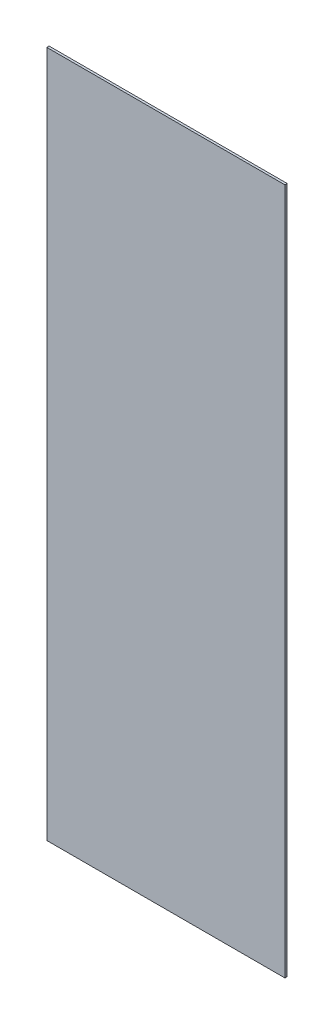
SolidWorks part; units mm, degrees
material "PMMA(有机玻璃)"
ref_plane "前视" through (0, 0, 0) normal (0, 0, 1) x (1, 0, 0)
ref_plane "上视" through (0, 0, 0) normal (0, 1, 0) x (1, 0, 0)
ref_plane "右视" through (0, 0, 0) normal (1, 0, 0) x (0, 0, -1)
sketch "草图1" plane through (0, 0, 0) normal (0, 0, 1) x (1, 0, 0)
  line L1 (-258.5, 745.5) -> (258.5, 745.5)
  line L2 (-258.5, 745.5) -> (-258.5, -745.5)
  line L3 (-258.5, -745.5) -> (258.5, -745.5)
  line L4 (258.5, 745.5) -> (258.5, -745.5)
  line L5 (-258.5, 745.5) -> (258.5, -745.5) construction
  line L6 (-258.5, -745.5) -> (258.5, 745.5) construction
  point P0 (0, 0)
  dimension "D1" = 1491
  dimension "D2" = 517
extrude "凸台-拉伸1" add sketch "草图1" along normal blind 5
hole_wizard "M5 间隙孔1" positions "草图3" profile "草图2" hole size "M5" standard "GB"
sketch "草图3" plane through (0, 0, 5) normal (0, 0, 1) x (1, 0, 0)
  line L0 (-427.5, 273) -> (-427.5, -273) construction
  line L1 (-427.5, -273) -> (427.5, -273) construction
  line L2 (0, 273) -> (0, -273) construction
  line L3 (427.5, 273) -> (-427.5, 273) construction
  line L5 (-427.5, 0) -> (427.5, 0) construction
  line L6 (427.5, -273) -> (427.5, 273) construction
  point P0 (-375, -261)
  point P46 (415.5, 250)
  point P48 (-415.5, 250)
  point P58 (-125, -261)
  point P59 (125, -261)
  point P61 (-125, 261)
  point P62 (125, 261)
  point P64 (-375, 261)
  point P88 (375, -261)
  point P89 (375, 261)
  point P108 (415.5, 0)
  point P109 (-415.5, 0)
  point P110 (415.5, -250)
  point P111 (-415.5, -250)
  dimension "D1" = 12
  dimension "D2" = 12
  dimension "D5" = 3
  dimension "D3" = 12
  dimension "D6" = 4
  dimension "D4" = 2
sketch "草图2" plane through (-375, -261, 5) normal (1, 0, 0) x (0, -1, 0)
  line L0 (0, 0) -> (0, 5)
  line L1 (0, 5) -> (2.75, 5)
  line L2 (2.75, 5) -> (2.75, 0)
  line L5 (2.75, 0) -> (0, 0)
  line L11 (0, -6.35) -> (0, 107.95) construction
  dimension "通孔孔直径" = 5.5
  dimension "通孔孔深度" = 5
